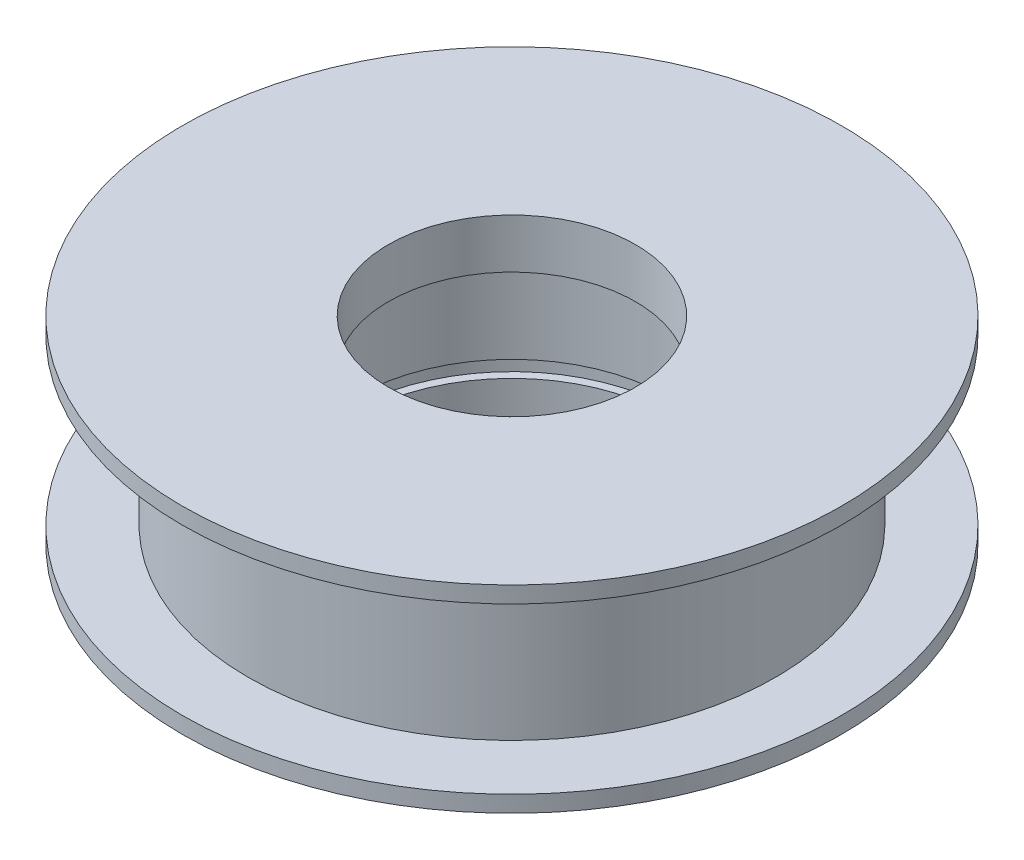
SolidWorks part; units mm, degrees
ref_plane "前视基准面" through (0, 0, 0) normal (0, 0, 1) x (1, 0, 0)
ref_plane "上视基准面" through (0, 0, 0) normal (0, 1, 0) x (1, 0, 0)
ref_plane "右视基准面" through (0, 0, 0) normal (1, 0, 0) x (0, 0, -1)
sketch "草图1" plane through (0, 0, 0) normal (0, 0, 1) x (1, 0, 0)
  line L0 (0, 22.4954) -> (0, -34.3351) construction
  line L1 (7.5, 3) -> (7.5, 0)
  line L2 (7.5, 0) -> (9.5, 0)
  line L3 (9.5, 0) -> (9.5, -6)
  line L4 (9.5, -9) -> (20, -9)
  line L5 (20, 3) -> (20, 2)
  line L6 (20, -9) -> (20, -8)
  line L7 (20, 2) -> (16, 2)
  line L8 (16, 2) -> (16, -8)
  line L9 (16, -8) -> (20, -8)
  line L10 (20, 3) -> (7.5, 3)
  line L11 (9.5, -7) -> (10, -7)
  line L12 (10, -7) -> (10, -6)
  line L13 (10, -6) -> (9.5, -6)
  line L14 (9.5, -7) -> (9.5, -9)
  dimension "D1" = 12
  dimension "D2" = 9.5
  dimension "D3" = 7.5
  dimension "D4" = 9
  dimension "D5" = 3
  dimension "D6" = 0.5
  dimension "D7" = 1
  dimension "D8" = 1
  dimension "D9" = 1
  dimension "D10" = 20
  dimension "D11" = 20
  dimension "D12" = 4
revolve "旋转1" add sketch "草图1" angle 360 about L0
